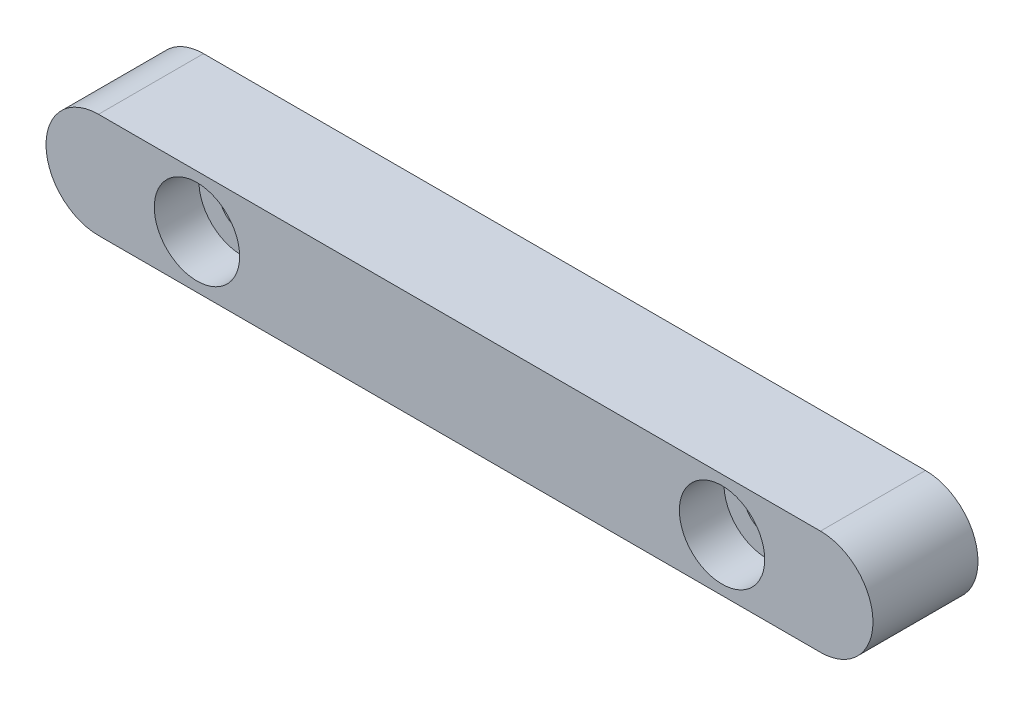
SolidWorks part; units mm, degrees
material "S45C"
ref_plane "Front Plane" through (0, 0, 0) normal (0, 0, 1) x (1, 0, 0)
ref_plane "Top Plane" through (0, 0, 0) normal (0, 1, 0) x (1, 0, 0)
ref_plane "Right Plane" through (0, 0, 0) normal (1, 0, 0) x (0, 0, -1)
sketch "Sketch1" plane through (0, 0, 0) normal (0, 0, 1) x (1, 0, 0)
  line L0 (-27.5, 0) -> (27.5, 0) construction
  line L1 (-27.5, 4) -> (27.5, 4)
  line L2 (-27.5, -4) -> (27.5, -4)
  arc A0 (-27.5, 4) -> (-27.5, -4) centre (-27.5, 0) ccw
  arc A1 (27.5, -4) -> (27.5, 4) centre (27.5, 0) ccw
  point P2 (0, 0)
  dimension "D1" = 8
  dimension "D2" = 55
extrude "Boss-Extrude1" add sketch "Sketch1" along normal blind 8
hole_wizard "CBORE for M3 Hex Socket Head Cap Screw1" positions "Sketch3" profile "Sketch2" counterbore size "M3" standard "Iso" end condition through all
sketch "Sketch3" plane through (0, 0, 8) normal (0, 0, 1) x (1, 0, 0)
  line L0 (0, 4) -> (0, 0) construction
  line L1 (27.5, 4) -> (-27.5, 4) construction
  point P0 (-20, 0)
  point P2 (20, 0)
  dimension "D1" = 40
sketch "Sketch2" plane through (-20, 0, 8) normal (1, 0, 0) x (0, -1, 0)
  line L0 (0, 0) -> (0, 8)
  line L1 (0, 8) -> (1.7, 8)
  line L3 (1.7, 8) -> (1.7, 3.4)
  line L4 (1.7, 3.4) -> (3.25, 3.4)
  line L5 (3.25, 3.4) -> (3.25, 0)
  line L7 (3.25, 0) -> (0, 0)
  line L11 (0, -6.35) -> (0, 107.95) construction
  dimension "通孔孔直径" = 3.4
  dimension "通孔孔深度" = 8
  dimension "柱形沉头孔直径" = 6.5
  dimension "柱形沉头孔深度" = 3.4
